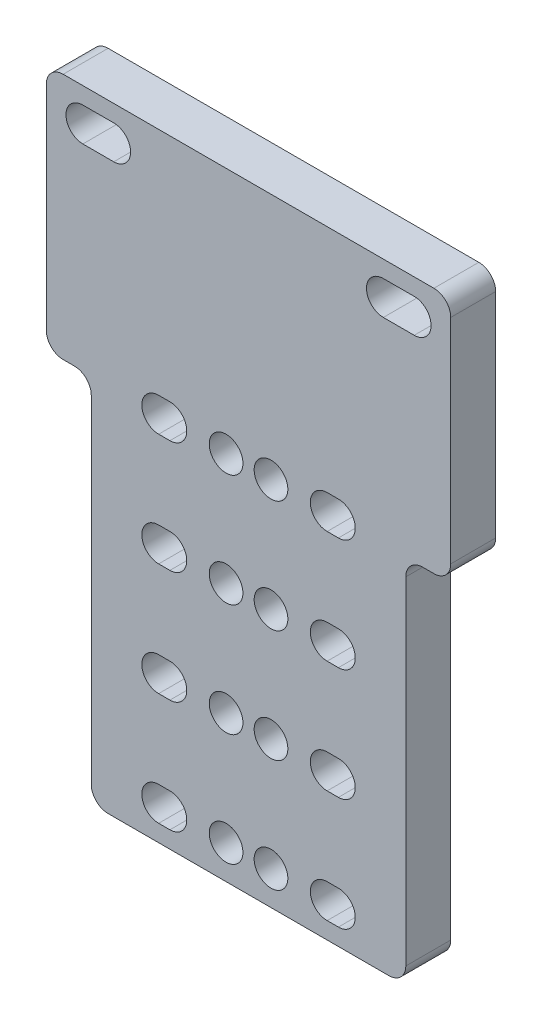
SolidWorks part; units mm, degrees
ref_plane "Front Plane" through (0, 0, 0) normal (0, 0, 1) x (1, 0, 0)
ref_plane "Top Plane" through (0, 0, 0) normal (0, 1, 0) x (1, 0, 0)
ref_plane "Right Plane" through (0, 0, 0) normal (1, 0, 0) x (0, 0, -1)
other "Configuration Table"
sketch "Sketch1" plane through (0, 0, 0) normal (0, 0, 1) x (1, 0, 0)
  line L1 (18, 27.5) -> (-18, 27.5)
  line L2 (18, 27.5) -> (18, -27.5)
  line L3 (18, -27.5) -> (-18, -27.5)
  line L4 (-18, 27.5) -> (-18, -27.5)
  line L5 (18, 27.5) -> (-18, -27.5) construction
  line L6 (18, -27.5) -> (-18, 27.5) construction
  point P0 (0, 0)
  dimension "D1" = 36
  dimension "D2" = 55
extrude "Boss-Extrude1" add sketch "Sketch1" along normal blind 4
sketch "Sketch2" plane through (0, 0, 4) normal (0, 0, 1) x (1, 0, 0)
  line L0 (0, -27.5) -> (0, 31.4566) construction
  line L1 (-18, -27.5) -> (18, -27.5) construction
  line L2 (-14.75, 24.5) -> (-12, 24.5) construction
  line L3 (-14.75, 26) -> (-12, 26)
  line L4 (-14.75, 23) -> (-12, 23)
  line L5 (12, 24.5) -> (14.75, 24.5) construction
  line L6 (12, 26) -> (14.75, 26)
  line L7 (12, 23) -> (14.75, 23)
  line L8 (-8, 5.5) -> (-7, 5.5) construction
  line L9 (-8, 7) -> (-7, 7)
  line L10 (-8, 4) -> (-7, 4)
  line L11 (7, 5.5) -> (8, 5.5) construction
  line L12 (7, 7) -> (8, 7)
  line L13 (7, 4) -> (8, 4)
  line L14 (-8, -4.5) -> (-7, -4.5) construction
  line L15 (-8, -3) -> (-7, -3)
  line L16 (-8, -6) -> (-7, -6)
  line L17 (7, -4.5) -> (8, -4.5) construction
  line L18 (7, -3) -> (8, -3)
  line L19 (7, -6) -> (8, -6)
  line L20 (-8, -14.5) -> (-7, -14.5) construction
  line L21 (-8, -13) -> (-7, -13)
  line L22 (-8, -16) -> (-7, -16)
  line L23 (7, -14.5) -> (8, -14.5) construction
  line L24 (7, -13) -> (8, -13)
  line L25 (7, -16) -> (8, -16)
  line L26 (-8, -24.5) -> (-7, -24.5) construction
  line L27 (-8, -23) -> (-7, -23)
  line L28 (-8, -26) -> (-7, -26)
  line L29 (7, -24.5) -> (8, -24.5) construction
  line L30 (7, -23) -> (8, -23)
  line L31 (7, -26) -> (8, -26)
  line L32 (-18, 5.5) -> (-14, 5.5)
  line L33 (-14, 5.5) -> (-14, -27.5)
  line L34 (14, 5.5) -> (14, -27.5)
  line L35 (18, 5.5) -> (14, 5.5)
  line L36 (-18, 27.5) -> (-18, -27.5)
  line L37 (-18, -27.5) -> (18, -27.5)
  line L38 (18, -27.5) -> (18, 27.5)
  line L39 (18, 27.5) -> (-18, 27.5)
  line L40 (-18, 26) -> (-18, -26)
  line L41 (-16.5, -27.5) -> (16.5, -27.5)
  line L42 (18, -26) -> (18, 26)
  line L43 (16.5, 27.5) -> (-16.5, 27.5)
  line L44 (-18, -26) -> (-18, -27.5)
  line L45 (-18, -27.5) -> (-16.5, -27.5)
  line L46 (16.5, -27.5) -> (18, -27.5)
  arc A0 (-14.75, 26) -> (-14.75, 23) centre (-14.75, 24.5) ccw
  arc A1 (-12, 23) -> (-12, 26) centre (-12, 24.5) ccw
  arc A2 (12, 26) -> (12, 23) centre (12, 24.5) ccw
  arc A3 (14.75, 23) -> (14.75, 26) centre (14.75, 24.5) ccw
  arc A4 (-8, 7) -> (-8, 4) centre (-8, 5.5) ccw
  arc A5 (-7, 4) -> (-7, 7) centre (-7, 5.5) ccw
  arc A6 (7, 7) -> (7, 4) centre (7, 5.5) ccw
  arc A7 (8, 4) -> (8, 7) centre (8, 5.5) ccw
  circle A8 centre (-2, 5.5) radius 1.5
  circle A9 centre (2, 5.5) radius 1.5
  circle A10 centre (-2, -4.5) radius 1.5
  circle A11 centre (2, -4.5) radius 1.5
  arc A12 (-8, -3) -> (-8, -6) centre (-8, -4.5) ccw
  arc A13 (-7, -6) -> (-7, -3) centre (-7, -4.5) ccw
  arc A14 (7, -3) -> (7, -6) centre (7, -4.5) ccw
  arc A15 (8, -6) -> (8, -3) centre (8, -4.5) ccw
  circle A16 centre (-2, -14.5) radius 1.5
  circle A17 centre (2, -14.5) radius 1.5
  arc A18 (-8, -13) -> (-8, -16) centre (-8, -14.5) ccw
  arc A19 (-7, -16) -> (-7, -13) centre (-7, -14.5) ccw
  arc A20 (7, -13) -> (7, -16) centre (7, -14.5) ccw
  arc A21 (8, -16) -> (8, -13) centre (8, -14.5) ccw
  circle A22 centre (-2, -24.5) radius 1.5
  circle A23 centre (2, -24.5) radius 1.5
  arc A24 (-8, -23) -> (-8, -26) centre (-8, -24.5) ccw
  arc A25 (-7, -26) -> (-7, -23) centre (-7, -24.5) ccw
  arc A26 (7, -23) -> (7, -26) centre (7, -24.5) ccw
  arc A27 (8, -26) -> (8, -23) centre (8, -24.5) ccw
  arc A28 (-18, 26) -> (-16.5, 27.5) centre (-16.5, 26) cw
  arc A29 (18, 26) -> (16.5, 27.5) centre (16.5, 26) ccw
  point P7 (-13.375, 24.5)
  point P12 (13.375, 24.5)
  point P19 (-7.5, 5.5)
  point P26 (7.5, 5.5)
  point P37 (-7.5, -4.5)
  point P45 (7.5, -4.5)
  point P56 (-7.5, -14.5)
  point P63 (7.5, -14.5)
  point P74 (-7.5, -24.5)
  point P81 (7.5, -24.5)
  line M1 (-18, 27.5) -> (-18, -27.5)
  line M2 (-18, -27.5) -> (18, -27.5)
  line M3 (18, -27.5) -> (18, 27.5)
  dimension "D1" = 1.5
  dimension "D2" = 1.5
  dimension "D3" = 24
  dimension "D5" = 1.5
  dimension "D6" = 3
  dimension "D7" = 3
  dimension "D8" = 1.5
  dimension "D14" = 1.5
  dimension "D15" = 1.5
  dimension "D16" = 1.5
  dimension "D4" = 29.5
  dimension "D9" = 4
  dimension "D10" = 5
  dimension "D11" = 16
  dimension "D12" = 4
  dimension "D18" = 10
  dimension "D19" = 28
  dimension "D13" = 0
extrude "Cut-Extrude1" cut sketch "Sketch2" against normal blind 4 contours L4 A1 L3 A0 | L7 A3 L6 A2 | L10 A5 L9 A4 | A8 | A9 | L13 A7 L12 A6 | L19 A15 L18 A14 | A11 | A10 | L16 A13 L15 A12 | L22 A19 L21 A18 | L28 A25 L27 A24 | A16 | A22 | A17 | A23 | L31 A27 L30 A26 | L33 L32 M1 M2 | L35 L34 M3 M2 | A20 L25 A21 L24
fillet "Fillet1" radius 1.5 6 edges at (-14, -27.5, 2) (14, -27.5, 2) (18, 5.5, 2) (-18, 5.5, 2) (18, 27.5, 2) (-18, 27.5, 2)
sketch "Sketch3" plane through (0, 0, 4) normal (0, 0, 1) x (1, 0, 0)
  line L0 (-15.5, 5.5) -> (-14, 5.5)
  line L1 (-14, 5.5) -> (-14, 4) construction
  line L2 (14, 4) -> (14, 5.5)
  line L4 (14, 5.5) -> (15.5, 5.5)
  arc A0 (-14, 4) -> (-15.5, 5.5) centre (-15.5, 4) ccw
  arc A1 (15.5, 5.5) -> (14, 4) centre (15.5, 4) ccw
  point P9 (-14, 5.5)
  point P16 (14, 5.5)
  dimension "D1" = 1.5
  dimension "D4" = 1.5
  dimension "D2" = 1.5
  dimension "D3" = 1.5
extrude "Boss-Extrude2" add sketch "Sketch3" against normal up to surface (4 mm away) contours L1 L0 A0 | A1 L2 L4 up to face at (-0.5, -14.5, 0)
